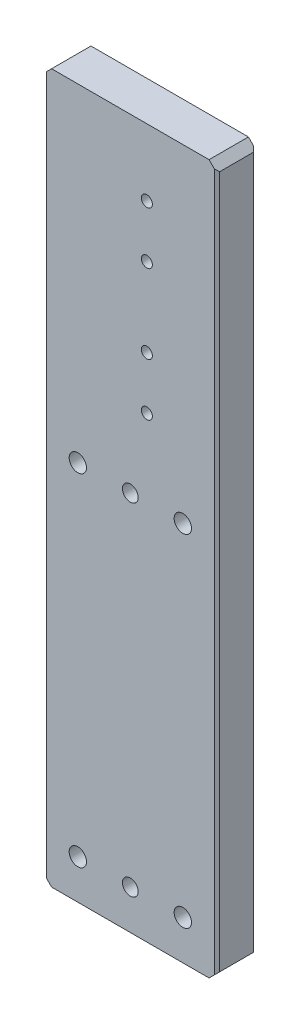
SolidWorks part; units mm, degrees
material "45"
ref_plane "Front Plane" through (0, 0, 0) normal (0, 0, 1) x (1, 0, 0)
ref_plane "Top Plane" through (0, 0, 0) normal (0, 1, 0) x (1, 0, 0)
ref_plane "Right Plane" through (0, 0, 0) normal (1, 0, 0) x (0, 0, -1)
sketch "Sketch1" plane through (0, 0, 0) normal (0, 0, 1) x (1, 0, 0)
  line L1 (0, 0) -> (66, 0)
  line L2 (0, 0) -> (0, 160)
  line L3 (0, 160) -> (66, 160)
  line L4 (66, 0) -> (66, 160)
  dimension "D1" = 66
  dimension "D2" = 160
extrude "Boss-Extrude1" add sketch "Sketch1" along normal blind 15
hole_wizard "CBORE for M6 Hex Socket Head Cap Screw1" positions "Sketch3" profile "Sketch2" counterbore size "M6" standard "Iso" end condition through all
sketch "Sketch3" plane through (0, 0, 0) normal (0, 0, -1) x (-1, 0, 0)
  line L0 (-66, 80) -> (0, 80) construction
  line L1 (-66, 0) -> (-66, 160) construction
  line L2 (0, 160) -> (0, 0) construction
  line L4 (-66, 160) -> (0, 160) construction
  line L5 (-33, 0) -> (-33, 160) construction
  line L6 (0, 0) -> (-66, 0) construction
  point P0 (-53, 15)
  point P2 (-13, 15)
  point P4 (-53, 145)
  point P6 (-13, 145)
  dimension "D1" = 15
  dimension "D2" = 40
sketch "Sketch2" plane through (53, 15, 0) normal (1, 0, 0) x (0, 1, 0)
  line L0 (0, 0) -> (0, 15)
  line L1 (0, 15) -> (3.3, 15)
  line L3 (3.3, 15) -> (3.3, 6.4)
  line L4 (3.3, 6.4) -> (5.5, 6.4)
  line L5 (5.5, 6.4) -> (5.5, 0)
  line L7 (5.5, 0) -> (0, 0)
  line L11 (0, -6.35) -> (0, 107.95) construction
  dimension "通孔孔直径" = 6.6
  dimension "通孔孔深度" = 15
  dimension "柱形沉头孔直径" = 11
  dimension "柱形沉头孔深度" = 6.4
other "Move Face1" face at (33, 160, 7.5) parameters "D1"=110
hole_wizard "M5 Tapped Hole1" positions "Sketch5" profile "Sketch4" tap size "M5" standard "Gb" end condition through all
sketch "Sketch5" plane through (0, 0, 0) normal (0, 0, -1) x (-1, 0, 0)
  line L0 (-39.3, 244.5) -> (-39.3, 224.5) construction
  line L2 (-39.3, 194.5) -> (-39.3, 174.5) construction
  circle A3 centre (-39.3, 174.5) radius 2.75 construction
  circle A4 centre (-39.3, 244.5) radius 2.75 construction
  point P0 (-39.3, 244.5)
  point P15 (-39.3, 174.5)
  point P30 (-39.3, 224.5)
  point P32 (-39.3, 194.5)
  dimension "D1" = 20
cosmetic thread "Hole thread 2" parameters "D2"=5
cosmetic thread "Hole thread 6" parameters "D2"=5
sketch "Sketch4" plane through (39.3, 244.5, 0) normal (1, 0, 0) x (0, 1, 0)
  line L0 (0, 0) -> (0, 15)
  line L1 (0, 15) -> (2.1, 15)
  line L2 (2.1, 15) -> (2.1, 0)
  line L5 (2.1, 0) -> (0, 0)
  line L11 (0, -6.35) -> (0, 107.95) construction
  dimension "通孔螺纹孔钻头直径" = 4.2
  dimension "通孔螺纹孔钻头深度" = 15
cosmetic thread "Hole thread 7" parameters "D2"=5
cosmetic thread "Hole thread 8" parameters "D2"=5
sketch "Sketch6" plane through (0, 0, 0) normal (0, 0, -1) x (-1, 0, 0)
  circle A0 centre (-39.3, 244.5) radius 3.5
  circle A1 centre (-39.3, 174.5) radius 3.5
  dimension "D1" = 7
extrude "Cut-Extrude1" cut sketch "Sketch6" against normal blind 1.6
chamfer "Chamfer2" distance 1 angle 45 4 edges at (0, 135, 15) (0, 135, 0) (66, 135, 0) (66, 135, 15)
chamfer "Chamfer1" distance 3 angle 45 4 edges at (0, 0, 7.5) (66, 0, 7.5) (0, 270, 7.5) (66, 270, 7.5)
sketch "Sketch12" plane through (0, 0, 0) normal (0, 0, -1) x (-1, 0, 0)
  line L0 (-13, 15) -> (-53, 15) construction
  line L2 (-13, 145) -> (-53, 145) construction
  circle A0 centre (-33, 145) radius 3
  circle A1 centre (-33, 15) radius 3
  dimension "D1" = 6
extrude "Cut-Extrude2" cut sketch "Sketch12" against normal through all
